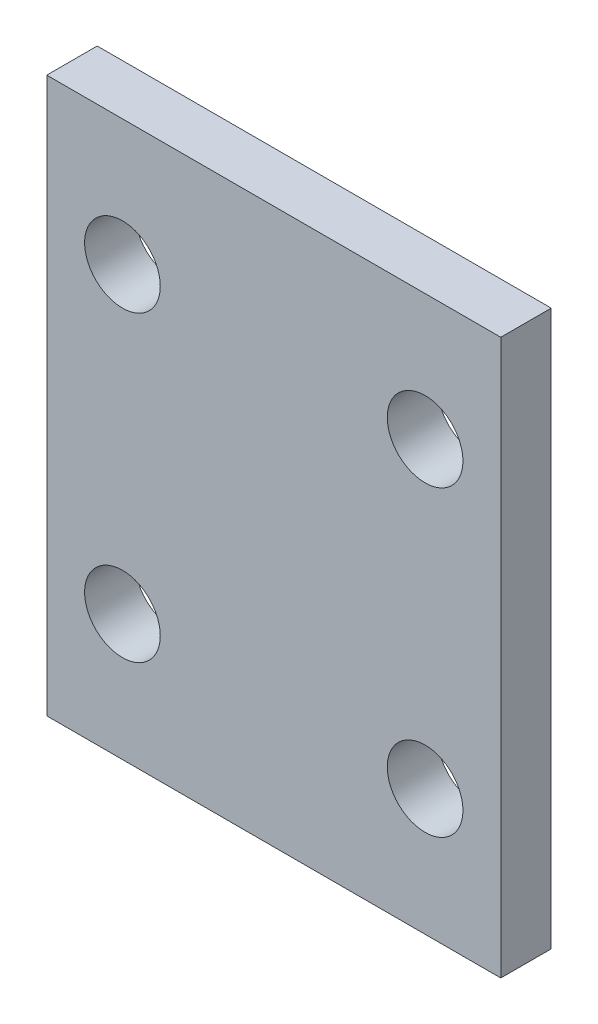
from build123d import *

# Parameters (mm, degrees)
SKETCH_1_W          = 100
SKETCH_1_H          = 120
EXTRUDE_1_DEPTH     = 10
CUT_EXTRUDE_1_DEPTH = 10
SKETCH_3_W          = 100
SKETCH_3_H          = 120
CUT_EXTRUDE_2_DEPTH = 10


with BuildPart() as part:
    # 草图1 → 凸台-拉伸1 (new body)
    with BuildSketch(Plane.XY):
        with Locations((50, 60)):
            Rectangle(SKETCH_1_W, SKETCH_1_H)
    extrude(amount=EXTRUDE_1_DEPTH)

    # 草图2 → 切除-拉伸1 (cut)
    with BuildSketch(Plane.XY.offset(10)):
        with BuildLine():
            ThreePointArc((87.5, 90), (80, 97.5), (72.5, 90))
            Line((72.5, 90), (80, 90))
            Line((80, 90), (80, 82.5))
            ThreePointArc((80, 82.5), (85.303300859, 84.696699141), (87.5, 90))
        make_face()
        with BuildLine():
            Line((80, 90), (72.5, 90))
            ThreePointArc((72.5, 90), (74.696699141, 84.696699141), (80, 82.5))
            Line((80, 82.5), (80, 90))
        make_face()
        with BuildLine():
            ThreePointArc((27.5, 90), (14.696699141, 95.303300859), (20, 82.5))
            Line((20, 82.5), (20, 90))
            Line((20, 90), (27.5, 90))
        make_face()
        with BuildLine():
            Line((20, 90), (20, 82.5))
            ThreePointArc((20, 82.5), (25.303300859, 84.696699141), (27.5, 90))
            Line((27.5, 90), (20, 90))
        make_face()
        with BuildLine():
            ThreePointArc((27.5, 30), (25.303300859, 35.303300859), (20, 37.5))
            Line((20, 37.5), (20, 30))
            Line((20, 30), (27.5, 30))
        make_face()
        with BuildLine():
            Line((20, 30), (20, 37.5))
            ThreePointArc((20, 37.5), (14.696699141, 24.696699141), (27.5, 30))
            Line((27.5, 30), (20, 30))
        make_face()
        with BuildLine():
            ThreePointArc((80, 37.5), (74.696699141, 35.303300859), (72.5, 30))
            Line((72.5, 30), (80, 30))
            Line((80, 30), (80, 37.5))
        make_face()
        with BuildLine():
            Line((80, 30), (72.5, 30))
            ThreePointArc((72.5, 30), (80, 22.5), (87.5, 30))
            ThreePointArc((87.5, 30), (85.303300859, 35.303300859), (80, 37.5))
            Line((80, 37.5), (80, 30))
        make_face()
    extrude(amount=-CUT_EXTRUDE_1_DEPTH, mode=Mode.SUBTRACT)

    # 草图3 → 切除-拉伸2 (cut)
    with BuildSketch(Plane.XY.offset(10)):
        with Locations((50, 60)):
            Rectangle(SKETCH_3_W, SKETCH_3_H)
        Polygon((95, 60), (95, 5), (5, 5), (5, 115), (95, 115), align=None, mode=Mode.SUBTRACT)
    extrude(amount=-CUT_EXTRUDE_2_DEPTH, mode=Mode.SUBTRACT)


solid = part.part
